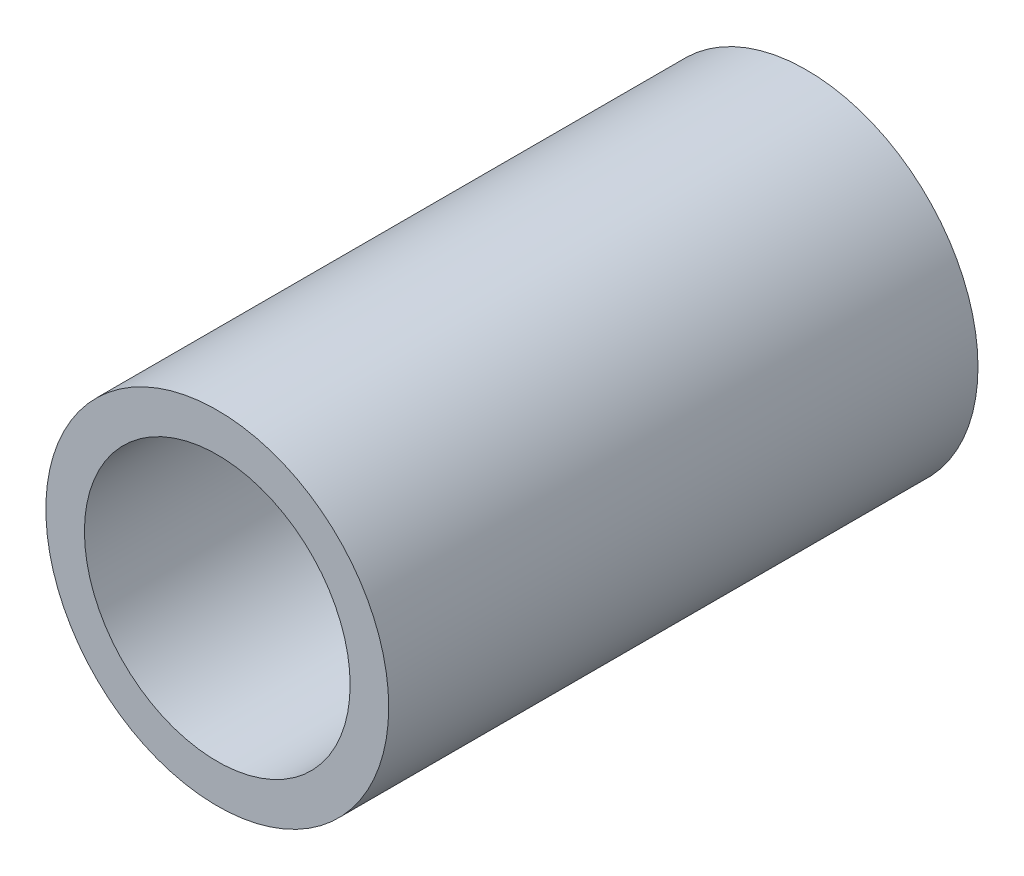
from build123d import *

# Parameters (mm, degrees)
SKETCH_1_R      = 16
SKETCH_1_R_2    = 12.4
EXTRUDE_1_DEPTH = 27.5


with BuildPart() as part:
    # 草图1 → 凸台-拉伸1 (new, symmetric)
    with BuildSketch(Plane.XY):
        Circle(SKETCH_1_R)
        Circle(SKETCH_1_R_2, mode=Mode.SUBTRACT)
    extrude(amount=EXTRUDE_1_DEPTH, both=True)


solid = part.part
